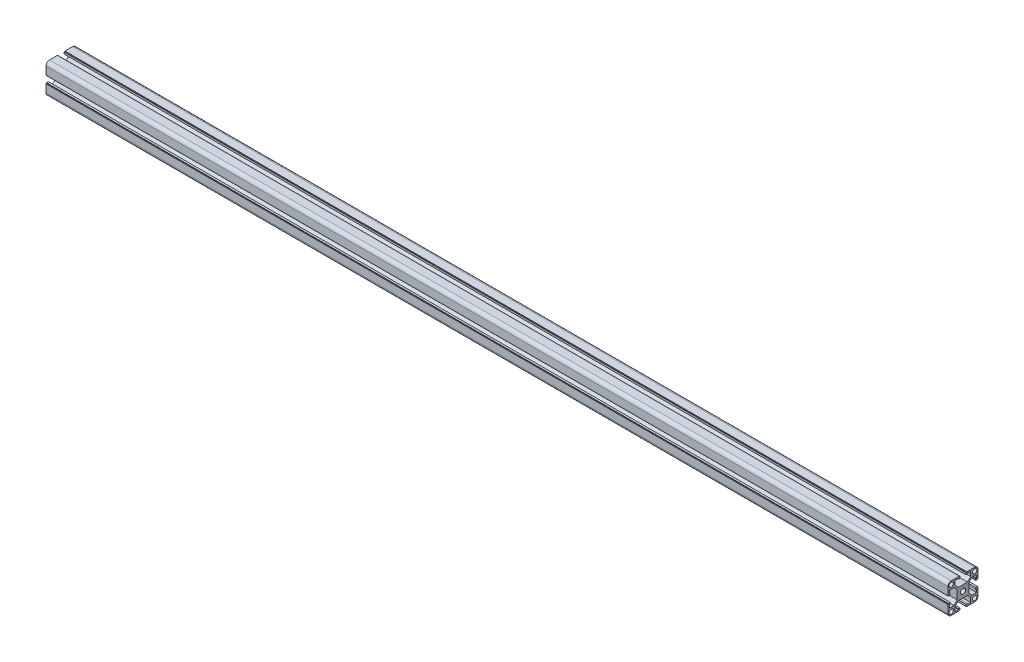
from build123d import *

# Parameters (mm, degrees)
SKETCH1_R                 = 3.4
SKETCH1_R_2               = 3
F_40_X_40W_X_R4_5_1_DEPTH = 1200


with BuildPart() as part:
    # Sketch1 → 铝型材 40 X 40W X R4.5(1) (new body)
    with BuildSketch(Plane(origin=(-600, 0, 0), x_dir=(0, 0, -1), z_dir=(1, 0, 0))):
        with BuildLine():
            Line((-5.1, 20), (-5.1, 19.5))
            Line((-5.1, 19.5), (-4.1, 19.5))
            Line((-4.1, 19.5), (-4.1, 17))
            Line((-4.1, 17), (-6.1, 17))
            Line((-6.1, 17), (-6.1, 18))
            Line((-6.1, 18), (-10.3, 18))
            Line((-10.3, 18), (-10.3, 12))
            Line((-10.3, 12), (-6, 7.7))
            Line((-6, 7.7), (6, 7.7))
            Line((6, 7.7), (10.3, 12))
            Line((10.3, 12), (10.3, 18))
            Line((10.3, 18), (6.1, 18))
            Line((6.1, 18), (6.1, 17))
            Line((6.1, 17), (4.1, 17))
            Line((4.1, 17), (4.1, 19.5))
            Line((4.1, 19.5), (5.1, 19.5))
            Line((5.1, 19.5), (5.1, 20))
            Line((5.1, 20), (15.5, 20))
            ThreePointArc((15.5, 20), (18.681980515, 18.681980515), (20, 15.5))
            Line((20, 15.5), (20, 5.1))
            Line((20, 5.1), (19.5, 5.1))
            Line((19.5, 5.1), (19.5, 4.1))
            Line((19.5, 4.1), (17, 4.1))
            Line((17, 4.1), (17, 6.1))
            Line((17, 6.1), (18, 6.1))
            Line((18, 6.1), (18, 10.3))
            Line((18, 10.3), (12, 10.3))
            Line((12, 10.3), (7.7, 6))
            Line((7.7, 6), (7.7, -6))
            Line((7.7, -6), (12, -10.3))
            Line((12, -10.3), (18, -10.3))
            Line((18, -10.3), (18, -6.1))
            Line((18, -6.1), (17, -6.1))
            Line((17, -6.1), (17, -4.1))
            Line((17, -4.1), (19.5, -4.1))
            Line((19.5, -4.1), (19.5, -5.1))
            Line((19.5, -5.1), (20, -5.1))
            Line((20, -5.1), (20, -15.5))
            ThreePointArc((20, -15.5), (18.681980515, -18.681980515), (15.5, -20))
            Line((15.5, -20), (5.1, -20))
            Line((5.1, -20), (5.1, -19.5))
            Line((5.1, -19.5), (4.1, -19.5))
            Line((4.1, -19.5), (4.1, -17))
            Line((4.1, -17), (6.1, -17))
            Line((6.1, -17), (6.1, -18))
            Line((6.1, -18), (10.3, -18))
            Line((10.3, -18), (10.3, -12))
            Line((10.3, -12), (6, -7.7))
            Line((6, -7.7), (-6, -7.7))
            Line((-6, -7.7), (-10.3, -12))
            Line((-10.3, -12), (-10.3, -18))
            Line((-10.3, -18), (-6.1, -18))
            Line((-6.1, -18), (-6.1, -17))
            Line((-6.1, -17), (-4.1, -17))
            Line((-4.1, -17), (-4.1, -19.5))
            Line((-4.1, -19.5), (-5.1, -19.5))
            Line((-5.1, -19.5), (-5.1, -20))
            Line((-5.1, -20), (-15.5, -20))
            ThreePointArc((-15.5, -20), (-18.681980515, -18.681980515), (-20, -15.5))
            Line((-20, -15.5), (-20, -5.1))
            Line((-20, -5.1), (-19.5, -5.1))
            Line((-19.5, -5.1), (-19.5, -4.1))
            Line((-19.5, -4.1), (-17, -4.1))
            Line((-17, -4.1), (-17, -6.1))
            Line((-17, -6.1), (-18, -6.1))
            Line((-18, -6.1), (-18, -10.3))
            Line((-18, -10.3), (-12, -10.3))
            Line((-12, -10.3), (-7.7, -6))
            Line((-7.7, -6), (-7.7, 6))
            Line((-7.7, 6), (-12, 10.3))
            Line((-12, 10.3), (-18, 10.3))
            Line((-18, 10.3), (-18, 6.1))
            Line((-18, 6.1), (-17, 6.1))
            Line((-17, 6.1), (-17, 4.1))
            Line((-17, 4.1), (-19.5, 4.1))
            Line((-19.5, 4.1), (-19.5, 5.1))
            Line((-19.5, 5.1), (-20, 5.1))
            Line((-20, 5.1), (-20, 15.5))
            ThreePointArc((-20, 15.5), (-18.681980515, 18.681980515), (-15.5, 20))
            Line((-15.5, 20), (-5.1, 20))
        make_face()
        Circle(SKETCH1_R, mode=Mode.SUBTRACT)
        with Locations((-15.556349186, 15.556349186)):
            Circle(SKETCH1_R_2, mode=Mode.SUBTRACT)
        with Locations((15.556349186, 15.556349186)):
            Circle(SKETCH1_R_2, mode=Mode.SUBTRACT)
        with Locations((15.556349186, -15.556349186)):
            Circle(SKETCH1_R_2, mode=Mode.SUBTRACT)
        with Locations((-15.556349186, -15.556349186)):
            Circle(SKETCH1_R_2, mode=Mode.SUBTRACT)
    extrude(amount=F_40_X_40W_X_R4_5_1_DEPTH)


solid = part.part
